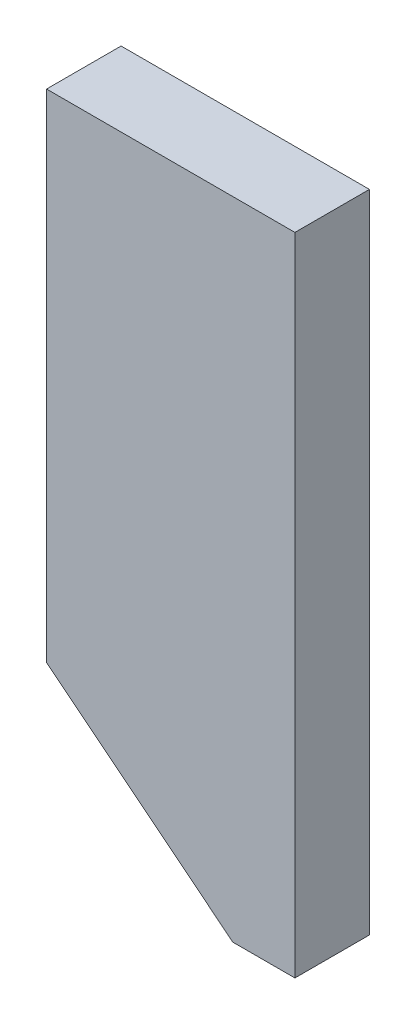
from build123d import *

# Parameters (mm, degrees)
SKETCH1_W           = 25
SKETCH1_H           = 310
EXTRUDE1_DEPTH      = 6
EXTRUDE3_DEPTH      = 6
SKETCH4_OUTSIDE_W   = 183.172
SKETCH4_OUTSIDE_H   = 378.172
SKETCH4_OUTSIDE_W_2 = 40
SKETCH4_OUTSIDE_H_2 = 128.082699231
CUT_EXTRUDE1_DEPTH  = 22


with BuildPart() as part:
    # Sketch1 → Extrude1 (new, symmetric)
    with BuildSketch(Plane.XY):
        Rectangle(SKETCH1_W, SKETCH1_H)
    extrude(amount=EXTRUDE1_DEPTH, both=True)

    # Sketch3 → Extrude3 (add, symmetric)
    with BuildSketch(Plane.XY):
        Polygon((-12.5, 155), (-72.5, 155), (-102.5, 131), (-102.5, 51), (-12.5, 51), align=None)
        Polygon((-12.5, -51), (-12.5, -155), (-72.5, -155), (-102.5, -131), (-102.5, -51), align=None)
    extrude(amount=EXTRUDE3_DEPTH, both=True)

    # Sketch4 outside → Cut-Extrude1 (cut)
    with BuildSketch(Plane.XY.offset(6)):
        with Locations((-45, 0)):
            Rectangle(SKETCH4_OUTSIDE_W, SKETCH4_OUTSIDE_H)
        with Locations((-82.5, -115.041349616)):
            Rectangle(SKETCH4_OUTSIDE_W_2, SKETCH4_OUTSIDE_H_2, mode=Mode.SUBTRACT)
    extrude(amount=-CUT_EXTRUDE1_DEPTH, mode=Mode.SUBTRACT)


solid = part.part
